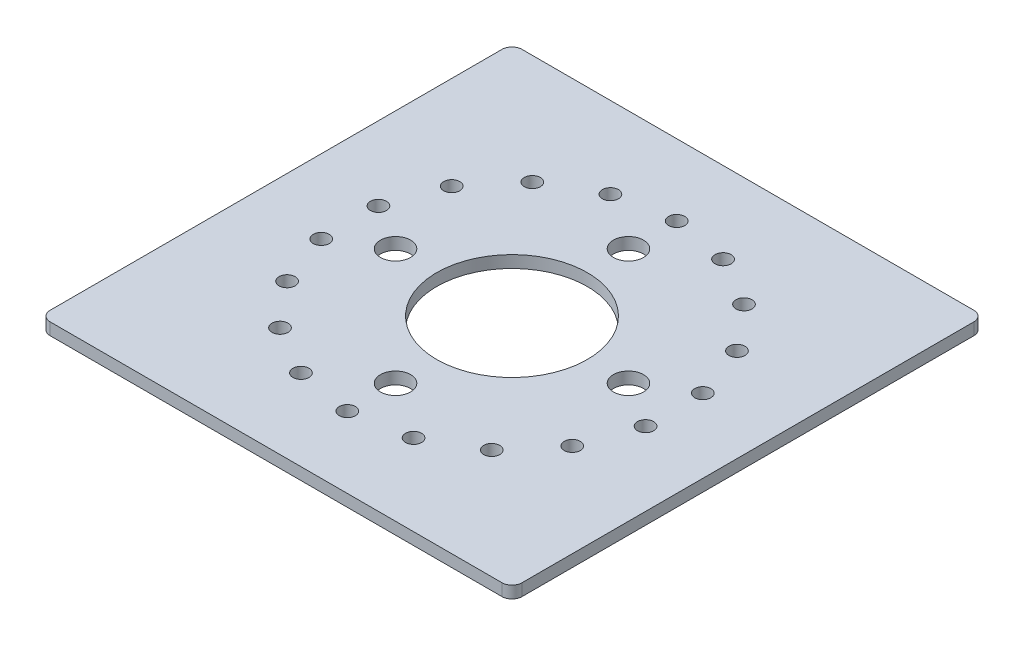
from build123d import *

# Parameters (mm, degrees)
SKETCH1_R                  = 75
BOSS_EXTRUDE1_DEPTH        = 12
F_16_0_16_DIAMETER_HOLE1_D = 16
F_30_DIAMETER_HOLE2_D      = 30


with BuildPart() as part:
    # Sketch1 → Boss-Extrude1 (new body)
    with BuildSketch(Plane(origin=(0, 0, 0), x_dir=(1, 0, 0), z_dir=(0, 1, 0))):
        with BuildLine():
            Line((225, -235), (-225, -235))
            ThreePointArc((-225, -235), (-232.071067812, -232.071067812), (-235, -225))
            Line((-235, -225), (-235, 225))
            ThreePointArc((-235, 225), (-232.071067812, 232.071067812), (-225, 235))
            Line((-225, 235), (225, 235))
            ThreePointArc((225, 235), (232.071067812, 232.071067812), (235, 225))
            Line((235, 225), (235, -225))
            ThreePointArc((235, -225), (232.071067812, -232.071067812), (225, -235))
        make_face()
        with Locations(Location((0, 0, 0), (0, 0, 270))):
            Circle(SKETCH1_R, mode=Mode.SUBTRACT)
    extrude(amount=BOSS_EXTRUDE1_DEPTH)

    # Ø16.0 (16) Diameter Hole1 (through all)
    with Locations(Plane(origin=(0, 12, 0), x_dir=(1, 0, 0), z_dir=(0, 1, 0))):
        with Locations((0, 164), (56.091303505, 154.109589809), (105.417167989, 125.631288672), (142.028166221, 82), (161.508471494, 28.478301137), (161.508471494, -28.478301137), (142.028166221, -82), (105.417167989, -125.631288672), (56.091303505, -154.109589809), (0, -164), (-56.091303505, -154.109589809), (-105.417167989, -125.631288672), (-142.028166221, -82), (-161.508471494, -28.478301137), (-161.508471494, 28.478301137), (-142.028166221, 82), (-105.417167989, 125.631288672), (-56.091303505, 154.109589809)):
            Hole(F_16_0_16_DIAMETER_HOLE1_D / 2)

    # Ø30 Diameter Hole2 (through all)
    with Locations(Plane(origin=(0, 12, 0), x_dir=(1, 0, 0), z_dir=(0, 1, 0))):
        with Locations((0, 116), (116, 0), (0, -116), (-116, 0)):
            Hole(F_30_DIAMETER_HOLE2_D / 2)


solid = part.part
